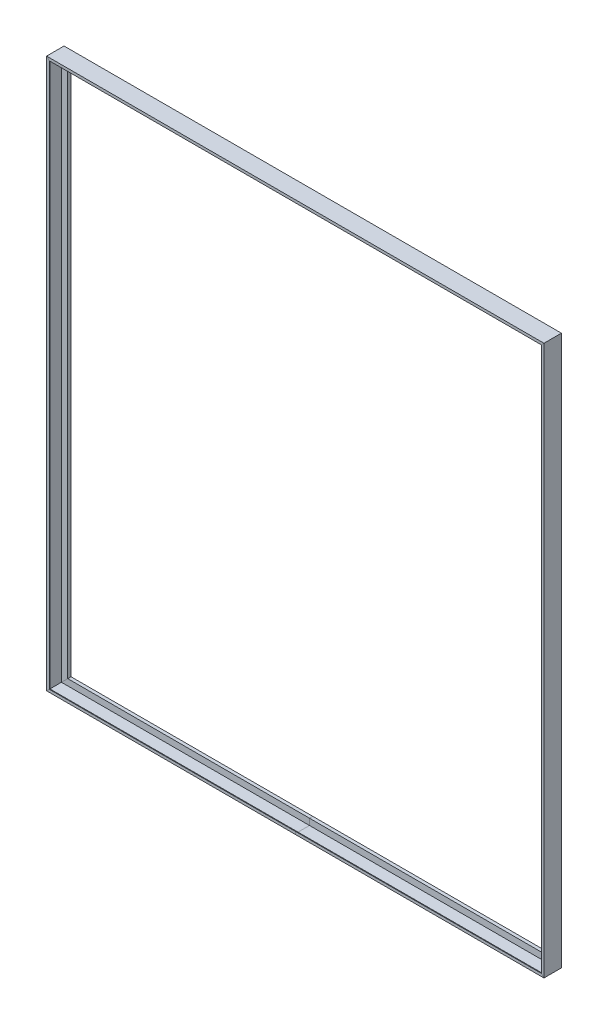
from build123d import *


with BuildPart() as part:
    # 扫描4: sweep along a path in 草图1
    with BuildLine(Plane.XY) as sweep_4_path:
        Line((-570, 630), (570, 630))
        Line((570, 630), (570, -630))
        Line((570, -630), (-570, -630))
        Line((-570, -630), (-570, 630))
    # 草图5 → 扫描4 (sweep)
    with BuildSketch(Plane(origin=(0, 0, 0), x_dir=(0, 0, -1), z_dir=(1, 0, 0))):
        Polygon((-40, -630), (0, -630), (0, -627.645553376), (-0.5, -627), (-1, -627), (-1, -628.5), (-6.5, -628.5), (-6.5, -615), (-1, -615), (-1, -617), (-0.5, -617), (0, -616.354446624), (0, -614), (-7.5, -614), (-7.5, -628.5), (-38.5, -628.5), (-38.5, -623.8), (-40, -623.8), align=None)
    sweep(path=sweep_4_path.line, transition=Transition.RIGHT)


solid = part.part
